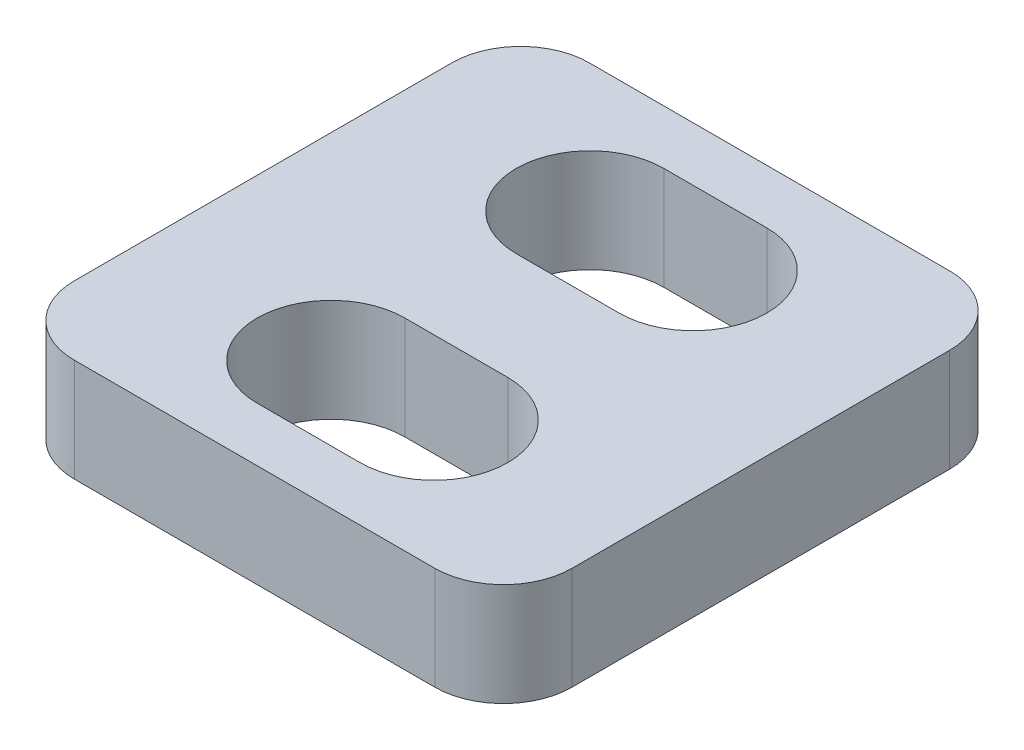
from build123d import *

# Parameters (mm, degrees)
SKETCH_1_W          = 14.5
SKETCH_1_H          = 15
EXTRUDE_1_DEPTH     = 3
CUT_EXTRUDE_1_DEPTH = 10
FILLET_1_R          = 2


with BuildPart() as part:
    # 草图1 → 凸台-拉伸1 (new body)
    with BuildSketch(Plane(origin=(0, 0, 0), x_dir=(1, 0, 0), z_dir=(0, 1, 0))):
        Rectangle(SKETCH_1_W, SKETCH_1_H)
    extrude(amount=EXTRUDE_1_DEPTH)

    # 草图4 → 切除-拉伸1 (cut)
    with BuildSketch(Plane.XZ):
        with BuildLine():
            Line((1.5, -5.922481842), (-1.5, -5.922481842))
            ThreePointArc((-1.5, -5.922481842), (-3.65, -3.772481842), (-1.5, -1.622481842))
            Line((-1.5, -1.622481842), (1.5, -1.622481842))
            ThreePointArc((1.5, -1.622481842), (3.65, -3.772481842), (1.5, -5.922481842))
        make_face()
        with BuildLine():
            Line((1.5, 5.922481842), (-1.5, 5.922481842))
            ThreePointArc((-1.5, 5.922481842), (-3.65, 3.772481842), (-1.5, 1.622481842))
            Line((-1.5, 1.622481842), (1.5, 1.622481842))
            ThreePointArc((1.5, 1.622481842), (3.65, 3.772481842), (1.5, 5.922481842))
        make_face()
    extrude(amount=-CUT_EXTRUDE_1_DEPTH, mode=Mode.SUBTRACT)

    # 圆角1
    fillet_1_edges = [part.edges().sort_by_distance(p)[0] for p in [
        (7.25, 1.5, 7.5),
        (-7.25, 1.5, 7.5),
        (-7.25, 1.5, -7.5),
        (7.25, 1.5, -7.5),
    ]]
    fillet(fillet_1_edges, radius=FILLET_1_R)


solid = part.part
